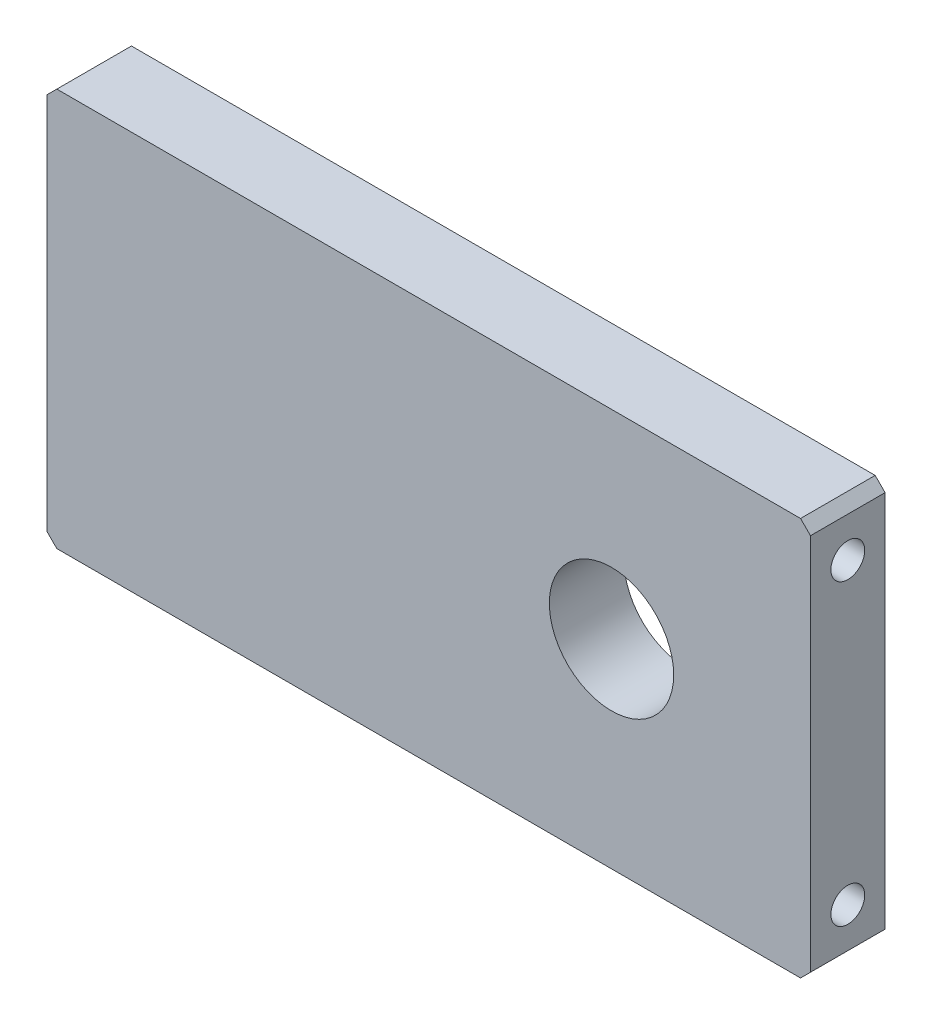
SolidWorks part; units mm, degrees
ref_plane "前视基准面" through (0, 0, 0) normal (0, 0, 1) x (1, 0, 0)
ref_plane "上视基准面" through (0, 0, 0) normal (0, 1, 0) x (1, 0, 0)
ref_plane "右视基准面" through (0, 0, 0) normal (1, 0, 0) x (0, 0, -1)
sketch "草图1" plane through (0, 0, 0) normal (0, 0, 1) x (1, 0, 0)
  line L1 (-76.75, 40) -> (76.75, 40)
  line L2 (-76.75, 40) -> (-76.75, -40)
  line L3 (-76.75, -40) -> (76.75, -40)
  line L4 (76.75, 40) -> (76.75, -40)
  line L5 (-76.75, 40) -> (76.75, -40) construction
  line L6 (-76.75, -40) -> (76.75, 40) construction
  point P0 (0, 0)
  dimension "D1" = 153.5
  dimension "D2" = 80
extrude "凸台-拉伸1" add sketch "草图1" along normal mid plane 15
hole_wizard "Ø25.0 (25) 直径孔1" positions "草图3" profile "草图2" hole size "Ø25.0" standard "ISO" end condition through all
sketch "草图3" plane through (0, 0, 7.5) normal (0, 0, 1) x (1, 0, 0)
  line L0 (76.75, -40) -> (76.75, 40) construction
  line L1 (-76.75, -40) -> (76.75, -40) construction
  point P0 (36.75, 0)
  dimension "D1" = 40
  dimension "D2" = 40
sketch "草图2" plane through (36.75, 0, 7.5) normal (1, 0, 0) x (0, -1, 0)
  line L0 (0, 0) -> (0, 15)
  line L1 (0, 15) -> (12.5, 15)
  line L2 (12.5, 15) -> (12.5, 0)
  line L5 (12.5, 0) -> (0, 0)
  line L11 (0, -6.35) -> (0, 107.95) construction
  dimension "通孔孔直径" = 25
  dimension "通孔孔深度" = 15
hole_wizard "M8 螺纹孔1" positions "草图5" profile "草图4" tap size "M8" standard "ISO"
sketch "草图5" plane through (76.75, 0, 0) normal (1, 0, 0) x (0, 0, -1)
  line L0 (-7.5, -40) -> (7.5, -40) construction
  point P0 (0, 30)
  point P2 (0, -30)
  dimension "D1" = 10
  dimension "D2" = 60
sketch "草图4" plane through (76.75, 30, 0) normal (0, 1, 0) x (0, 0, -1)
  line L0 (0, 0) -> (0, 21.7929)
  line L1 (0, 21.7929) -> (3.4, 19.75)
  line L2 (3.4, 19.75) -> (3.4, 0)
  line L5 (3.4, 0) -> (0, 0)
  line L10 (0, 21.7929) -> (-3.4, 19.75) construction
  line L11 (0, -6.35) -> (0, 107.95) construction
  dimension "螺纹孔钻头直径" = 6.8
  dimension "螺纹孔钻头深度" = 19.75
  dimension "导头角度" = 118
cosmetic thread "孔螺蚊线1" parameters "D1"=16, "D2"=8
cosmetic thread "孔螺蚊线2" parameters "D1"=16, "D2"=8
mirror "镜向1" about plane through (0, 0, 0) normal (1, 0, 0) of "M8 螺纹孔1"
chamfer "倒角1" distance 2 angle 45 4 edges at (-76.75, 40, 0) (-76.75, -40, 0) (76.75, -40, 0) (76.75, 40, 0)
